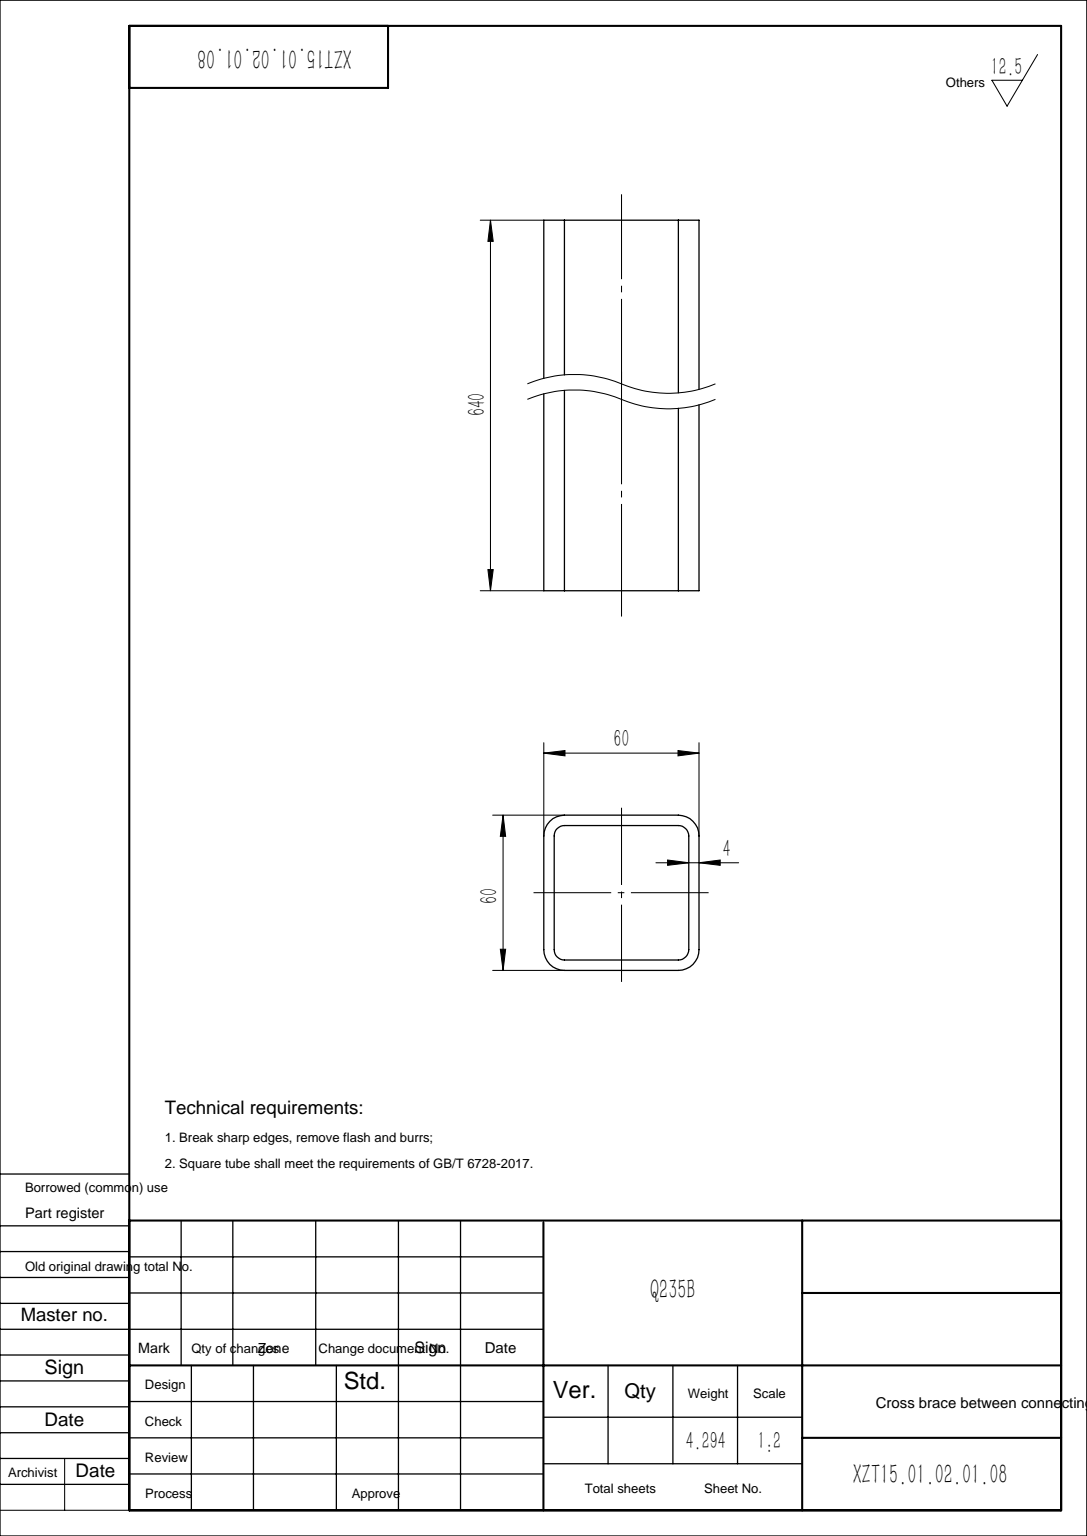
SolidWorks part; units mm, degrees
material "Q235B"
ref_plane "Front Plane" through (0, 0, 0) normal (0, 0, 1) x (1, 0, 0)
ref_plane "Top Plane" through (0, 0, 0) normal (0, 1, 0) x (1, 0, 0)
ref_plane "Right Plane" through (0, 0, 0) normal (1, 0, 0) x (0, 0, -1)
sketch "草图1" plane through (0, 0, 0) normal (0, 0, 1) x (1, 0, 0)
  line L0 (0, 0) -> (0, 640)
  dimension "D1" = 640
other "GB/T 6728-2002 square hollow section 60×60×4(1)"
ref_plane "Plane1" through (0, 0, 0) normal (0, 1, 0) x (-1, 0, 0)
sketch "Sketch1" plane through (0, 0, 0) normal (0, 1, 0) x (-1, 0, 0)
  line L0 (-22, -26) -> (22, -26)
  line L1 (-26, -22) -> (-26, 22)
  line L2 (22, 26) -> (-22, 26)
  line L3 (26, 22) -> (26, -22)
  line L4 (-22, -30) -> (22, -30)
  line L5 (-30, -22) -> (-30, 22)
  line L6 (22, 30) -> (-22, 30)
  line L7 (30, 22) -> (30, -22)
  arc A0 (30, 22) -> (22, 30) centre (22, 22) ccw
  arc A1 (22, -30) -> (30, -22) centre (22, -22) ccw
  arc A2 (-30, -22) -> (-22, -30) centre (-22, -22) ccw
  arc A3 (-22, 30) -> (-30, 22) centre (-22, 22) ccw
  arc A4 (-22, 26) -> (-26, 22) centre (-22, 22) ccw
  arc A5 (26, 22) -> (22, 26) centre (22, 22) ccw
  arc A6 (22, -26) -> (26, -22) centre (22, -22) ccw
  arc A7 (-26, -22) -> (-22, -26) centre (-22, -22) ccw
  point P0 (-30, 0)
  point P1 (30, 0)
  point P2 (0, 30)
  point P3 (0, -30)
  point P4 (0, 0)
  point P5 (-30, -30)
  point P6 (30, -30)
  point P7 (30, 30)
  point P8 (-30, 30)
  point P33 (0, 0)
  dimension "D1" = 8
  dimension "Thickness" = 4
  dimension "V_leg" = 60
